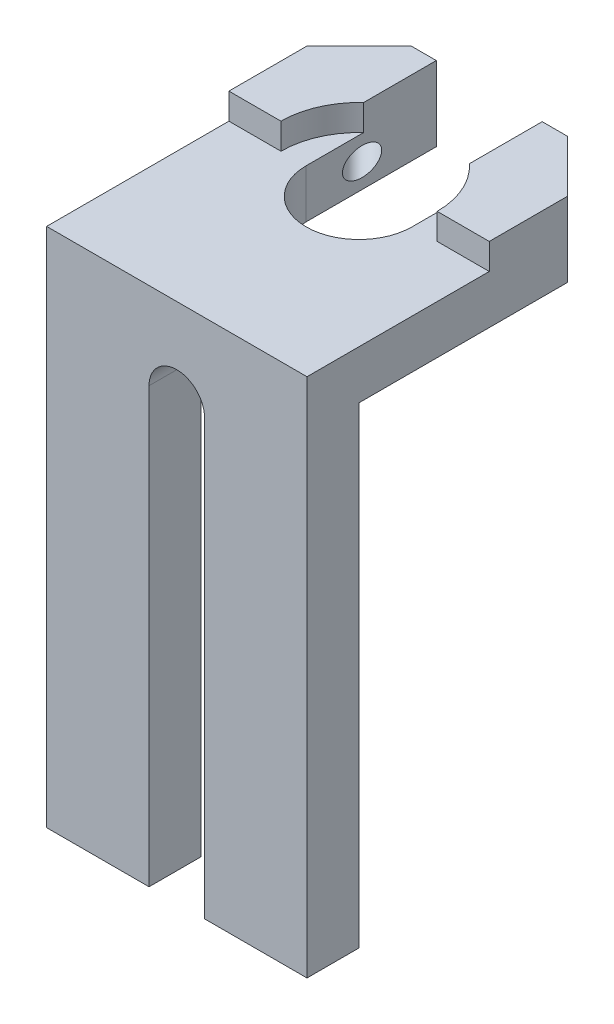
from build123d import *

# Parameters (mm, degrees)
BOSS_EXTRUDE1_DEPTH = 2.8
SKETCH3_W           = 4.45
SKETCH3_H           = 4.3
BOSS_EXTRUDE2_DEPTH = 1.5
SKETCH4_R           = 4.5
CUT_EXTRUDE2_DEPTH  = 10
BOSS_EXTRUDE3_DEPTH = 1.5
CUT_EXTRUDE5_DEPTH  = 12.445086282
SKETCH17_W          = 15
SKETCH17_H          = 30
BOSS_EXTRUDE4_DEPTH = 3
CUT_EXTRUDE6_DEPTH  = 233


with BuildPart() as part:
    # Sketch1 → Boss-Extrude1 (new body)
    with BuildSketch(Plane(origin=(0, 0, 0), x_dir=(1, 0, 0), z_dir=(0, 1, 0))):
        with BuildLine():
            Line((-3.05, 0), (-3.05, 7.5))
            Line((-3.05, 7.5), (-7.5, 7.5))
            Line((-7.5, 7.5), (-7.5, -7.5))
            Line((-7.5, -7.5), (7.5, -7.5))
            Line((7.5, -7.5), (7.5, 7.5))
            Line((7.5, 7.5), (3.05, 7.5))
            Line((3.05, 7.5), (3.05, 0))
            ThreePointArc((3.05, 0), (0, -3.05), (-3.05, 0))
        make_face()
    extrude(amount=BOSS_EXTRUDE1_DEPTH)

    # Sketch3 → Boss-Extrude2 (add)
    with BuildSketch(Plane(origin=(0, 2.8, 0), x_dir=(1, 0, 0), z_dir=(0, 1, 0))):
        with Locations((-5.275, 5.35)):
            Rectangle(SKETCH3_W, SKETCH3_H)
        with Locations((5.275, 5.35)):
            Rectangle(SKETCH3_W, SKETCH3_H)
    extrude(amount=BOSS_EXTRUDE2_DEPTH)

    # Sketch4 → Cut-Extrude2 (cut)
    with BuildSketch(Plane(origin=(0, 2.8, 0), x_dir=(1, 0, 0), z_dir=(0, 1, 0))):
        Circle(SKETCH4_R)
    extrude(amount=CUT_EXTRUDE2_DEPTH, mode=Mode.SUBTRACT)

    # Sketch5 → Boss-Extrude3 (add)
    with BuildSketch(Plane(origin=(0, 2.8, 0), x_dir=(1, 0, 0), z_dir=(0, 1, 0))):
        with BuildLine():
            Line((-7.5, 3.2), (-7.5, 0))
            Line((-7.5, 0), (-4.5, 0))
            ThreePointArc((-4.5, 0), (-4.152551193, 1.733873868), (-3.163858404, 3.2))
            Line((-3.163858404, 3.2), (-7.5, 3.2))
        make_face()
        with BuildLine():
            ThreePointArc((3.163858404, 3.2), (4.152551193, 1.733873868), (4.5, 0))
            Line((4.5, 0), (7.5, 0))
            Line((7.5, 0), (7.5, 3.2))
            Line((7.5, 3.2), (3.163858404, 3.2))
        make_face()
    extrude(amount=BOSS_EXTRUDE3_DEPTH)

    # Sketch14 → Cut-Extrude5 (cut, through all)
    with BuildSketch(Plane(origin=(0, 4.3, 0), x_dir=(1, 0, 0), z_dir=(0, 1, 0))):
        Polygon((4.5, 7.5), (7.5, 4.5), (7.5, 7.5), align=None)
        Polygon((-7.5, 7.5), (-4.5, 7.5), (-7.5, 4.5), align=None)
    extrude(amount=-CUT_EXTRUDE5_DEPTH, mode=Mode.SUBTRACT)

    # Sketch16 → M2 Tapped Hole1 (revolve, cut)
    with BuildSketch(Plane(origin=(5.914213562, 1.4, -6.085786438), x_dir=(-0.7071067811865475, 0, -0.7071067811865477), z_dir=(0, 1, 0))):
        Polygon((0, 0), (0, 8.480688495), (0.8, 8), (0.8, 0), align=None)
    m2_tapped_hole1 = revolve(axis=Axis((10.404341623, 1.4, -10.575914498), (-0.7071067811865477, 0, 0.7071067811865475)), mode=Mode.SUBTRACT)

    # Mirror1: M2 Tapped Hole1 across plane
    add(m2_tapped_hole1.mirror(Plane(origin=(0, 0, 0), x_dir=(0, 0, 1), z_dir=(1, 0, 0))), mode=Mode.SUBTRACT)

    # Sketch17 → Boss-Extrude4 (add)
    with BuildSketch(Plane.XY.offset(7.5)):
        with Locations((0, -12.2)):
            Rectangle(SKETCH17_W, SKETCH17_H)
    extrude(amount=BOSS_EXTRUDE4_DEPTH)

    # Sketch18 → Cut-Extrude6 (cut)
    with BuildSketch(Plane(origin=(0, 0, 7.5), x_dir=(-1, 0, 0), z_dir=(0, 0, -1))):
        with BuildLine():
            Line((-1.6, -27.2), (-1.6, -2.2))
            ThreePointArc((-1.6, -2.2), (0, -0.6), (1.6, -2.2))
            Line((1.6, -2.2), (1.6, -27.2))
            ThreePointArc((1.6, -27.2), (0, -28.8), (-1.6, -27.2))
        make_face()
    extrude(amount=-CUT_EXTRUDE6_DEPTH, mode=Mode.SUBTRACT)


solid = part.part
